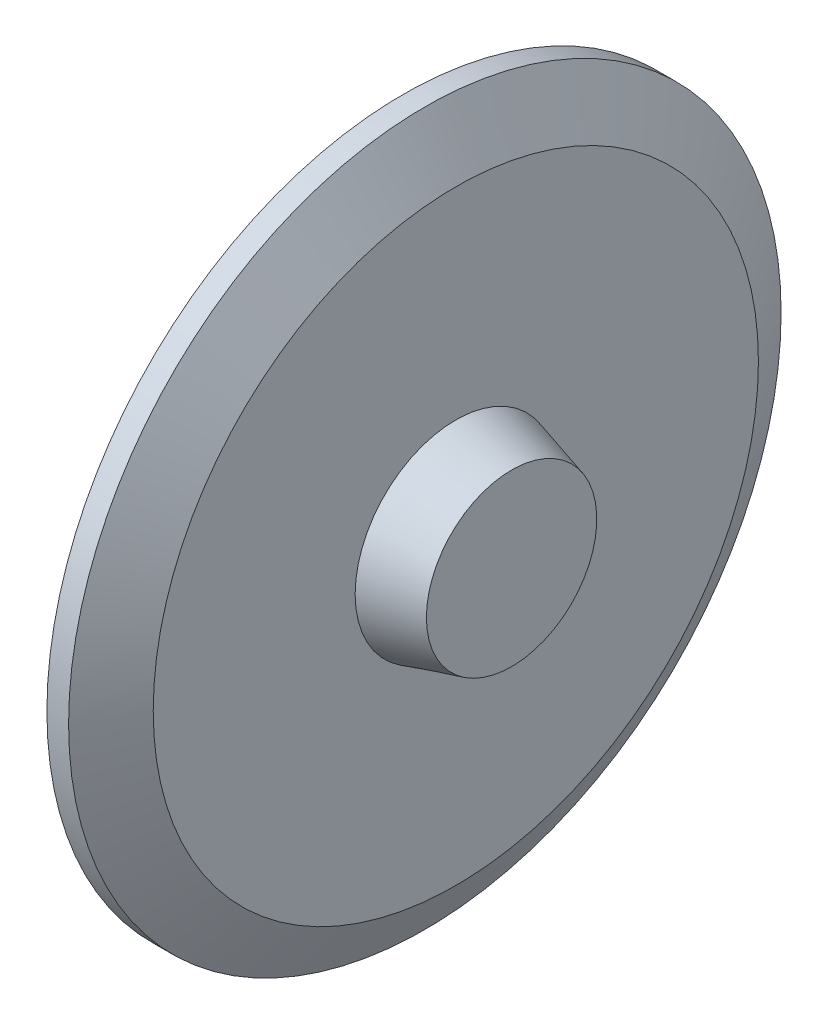
SolidWorks part; units mm, degrees
ref_plane "Front Plane" through (0, 0, 0) normal (0, 0, 1) x (1, 0, 0)
ref_plane "Top Plane" through (0, 0, 0) normal (0, 1, 0) x (1, 0, 0)
ref_plane "Right Plane" through (0, 0, 0) normal (1, 0, 0) x (0, 0, -1)
other "Configuration Table"
sketch "Sketch1" plane through (0, 0, 0) normal (0, 0, 1) x (1, 0, 0)
  line L0 (0, 0) -> (248.2545, 0) construction
  line L1 (0, 0) -> (0, 100)
  line L2 (0, 100) -> (4, 100)
  line L3 (4, 100) -> (4, 115)
  line L4 (11, 115) -> (21, 97.6795)
  line L5 (21, 97.6795) -> (21, 32.5)
  line L6 (21, 32.5) -> (39, 27.5)
  line L7 (39, 27.5) -> (39, 0)
  line L8 (4, 115) -> (11, 115)
  line L9 (0, 0) -> (39, 0)
  dimension "D1" = 230
  dimension "D2" = 200
  dimension "D3" = 17
  dimension "D4" = 7
  dimension "D5" = 60
  dimension "D6" = 4
  dimension "D7" = 65
  dimension "D8" = 55
  dimension "D9" = 39
revolve "Revolve1" add sketch "Sketch1" angle 360 about L0
